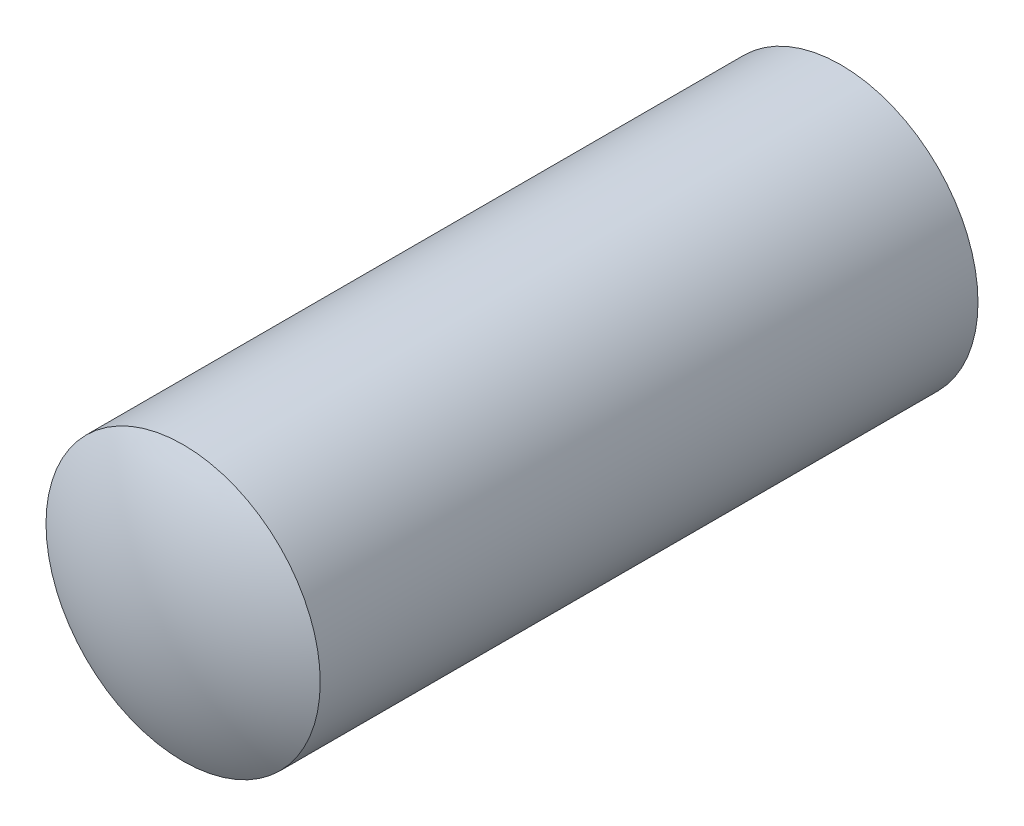
from build123d import *


with BuildPart() as part:
    # Logo3_bib1 → Revolve1 (revolve)
    with BuildSketch(Plane(origin=(0, 0, 0), x_dir=(-1, 0, 0), z_dir=(0, -1, 0))):
        with BuildLine():
            Line((0, 6), (0, -2))
            ThreePointArc((0, -2), (0.776457135, -1.897777479), (1.5, -1.598076211))
            Line((1.5, -1.598076211), (1.5, 5.598076211))
            ThreePointArc((1.5, 5.598076211), (0.776457135, 5.897777479), (0, 6))
        make_face()
    revolve(axis=Axis((0, 0, -47.537203702), (0, 0, 1)))


solid = part.part
